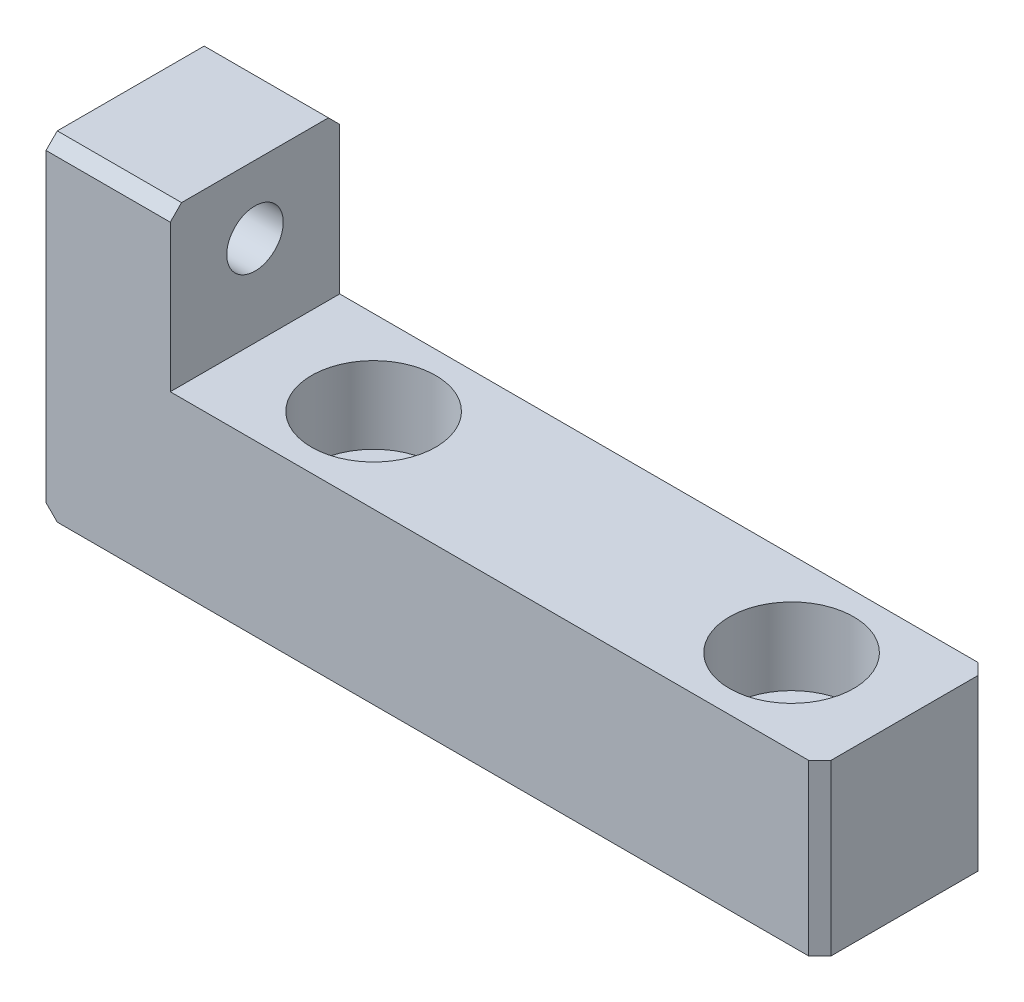
SolidWorks part; units mm, degrees
material "45#"
ref_plane "前基準面" through (0, 0, 0) normal (0, 0, 1) x (1, 0, 0)
ref_plane "上基準面" through (0, 0, 0) normal (0, 1, 0) x (1, 0, 0)
ref_plane "右基準面" through (0, 0, 0) normal (1, 0, 0) x (0, 0, -1)
sketch "草图1" plane through (0, 0, 0) normal (0, 1, 0) x (1, 0, 0)
  line L1 (-34.25, -7.5) -> (34.25, -7.5)
  line L2 (-34.25, -7.5) -> (-34.25, 7.5)
  line L3 (-34.25, 7.5) -> (34.25, 7.5)
  line L4 (34.25, -7.5) -> (34.25, 7.5)
  line L5 (-34.25, -7.5) -> (34.25, 7.5) construction
  line L6 (-34.25, 7.5) -> (34.25, -7.5) construction
  point P0 (0, 0)
  dimension "D1" = 68.5
  dimension "D2" = 15
extrude "凸台-拉伸1" add sketch "草图1" along normal mid plane 15
sketch "草图2" plane through (0, 7.5, 0) normal (0, 1, 0) x (1, 0, 0)
  line L0 (-34.25, -7.5) -> (34.25, -7.5) construction
  line L1 (-34.25, 7.5) -> (-23.25, 7.5)
  line L2 (-34.25, 7.5) -> (-34.25, -7.5)
  line L3 (-34.25, -7.5) -> (-23.25, -7.5)
  line L4 (-23.25, 7.5) -> (-23.25, -7.5)
  dimension "D1" = 11
extrude "凸台-拉伸2" add sketch "草图2" along normal blind 14
chamfer "倒角1" distance 1 angle 45 5 edges at (34.25, 0, -7.5) (34.25, 0, 7.5) (-34.25, -7.5, 0) (-28.75, 21.5, -7.5) (-28.75, 21.5, 7.5)
sketch "草图3" plane through (0, 7.5, 0) normal (0, 1, 0) x (1, 0, 0)
  line L0 (34.25, -6.5) -> (34.25, 6.5) construction
  point P0 (24.25, 0)
  point P2 (-12.75, 0)
  dimension "D1" = 37
  dimension "D2" = 10
hole_wizard "M6 六角圆柱头螺钉的柱形沉头孔1" positions "草图3" profile "草图4" counterbore size "M6" standard "GB" end condition through all
sketch "草图4" plane through (24.25, 7.5, 0) normal (1, 0, 0) x (0, 0, 1)
  line L0 (0, 0) -> (0, 15)
  line L1 (0, 15) -> (3.3, 15)
  line L3 (3.3, 15) -> (3.3, 6.8)
  line L4 (3.3, 6.8) -> (5.5, 6.8)
  line L5 (5.5, 6.8) -> (5.5, 0)
  line L7 (5.5, 0) -> (0, 0)
  line L11 (0, -6.35) -> (0, 107.95) construction
  dimension "通孔孔直径" = 6.6
  dimension "通孔孔深度" = 15
  dimension "柱形沉头孔直径" = 11
  dimension "柱形沉头孔深度" = 6.8
sketch "草图5" plane through (-34.25, 0, 0) normal (-1, 0, 0) x (0, 0, 1)
  line L1 (-6.5, 21.5) -> (6.5, 21.5) construction
  point P0 (0, 15.5)
  dimension "D1" = 6
hole_wizard "M6 螺纹孔1" positions "草图5" profile "草图6" tap size "M6" standard "GB" end condition through all
sketch "草图6" plane through (-34.25, 15.5, 0) normal (0, 1, 0) x (0, 0, 1)
  line L0 (0, 0) -> (0, 68.5)
  line L1 (0, 68.5) -> (2.5, 68.5)
  line L2 (2.5, 68.5) -> (2.5, 0)
  line L5 (2.5, 0) -> (0, 0)
  line L11 (0, -6.35) -> (0, 107.95) construction
  dimension "通孔螺纹孔钻头直径" = 5
  dimension "通孔螺纹孔钻头深度" = 68.5
cosmetic thread "孔螺纹线1" parameters "D2"=6
